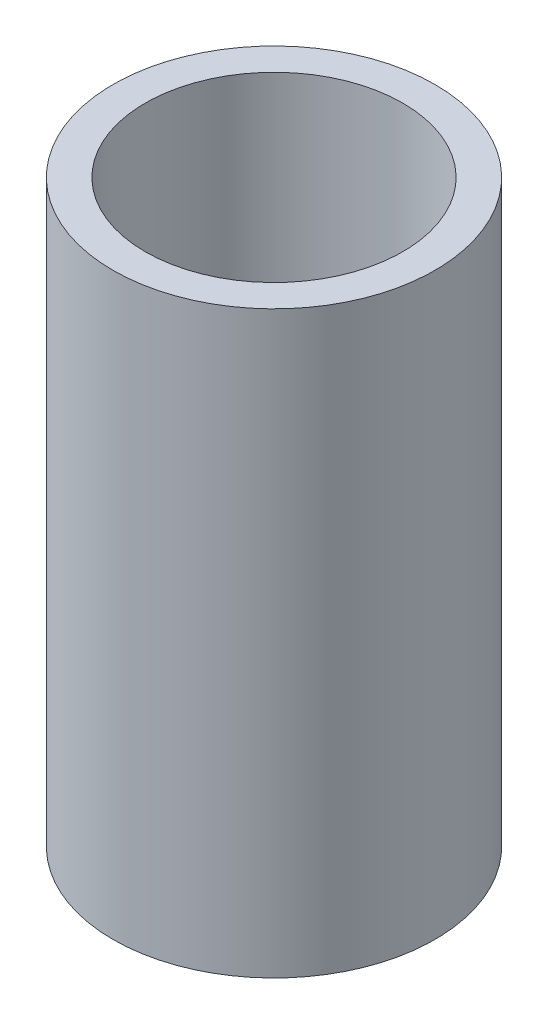
SolidWorks part; units mm, degrees
ref_plane "Front Plane" through (0, 0, 0) normal (0, 0, 1) x (1, 0, 0)
ref_plane "Top Plane" through (0, 0, 0) normal (0, 1, 0) x (1, 0, 0)
ref_plane "Right Plane" through (0, 0, 0) normal (1, 0, 0) x (0, 0, -1)
other "Configuration Table"
sketch "Sketch1" plane through (0, 0, 0) normal (0, 1, 0) x (1, 0, 0)
  circle A0 centre (0, 0) radius 8
  circle A1 centre (0, 0) radius 10
  dimension "D1" = 16
  dimension "D2" = 20
extrude "Boss-Extrude1" add sketch "Sketch1" along normal blind 36
